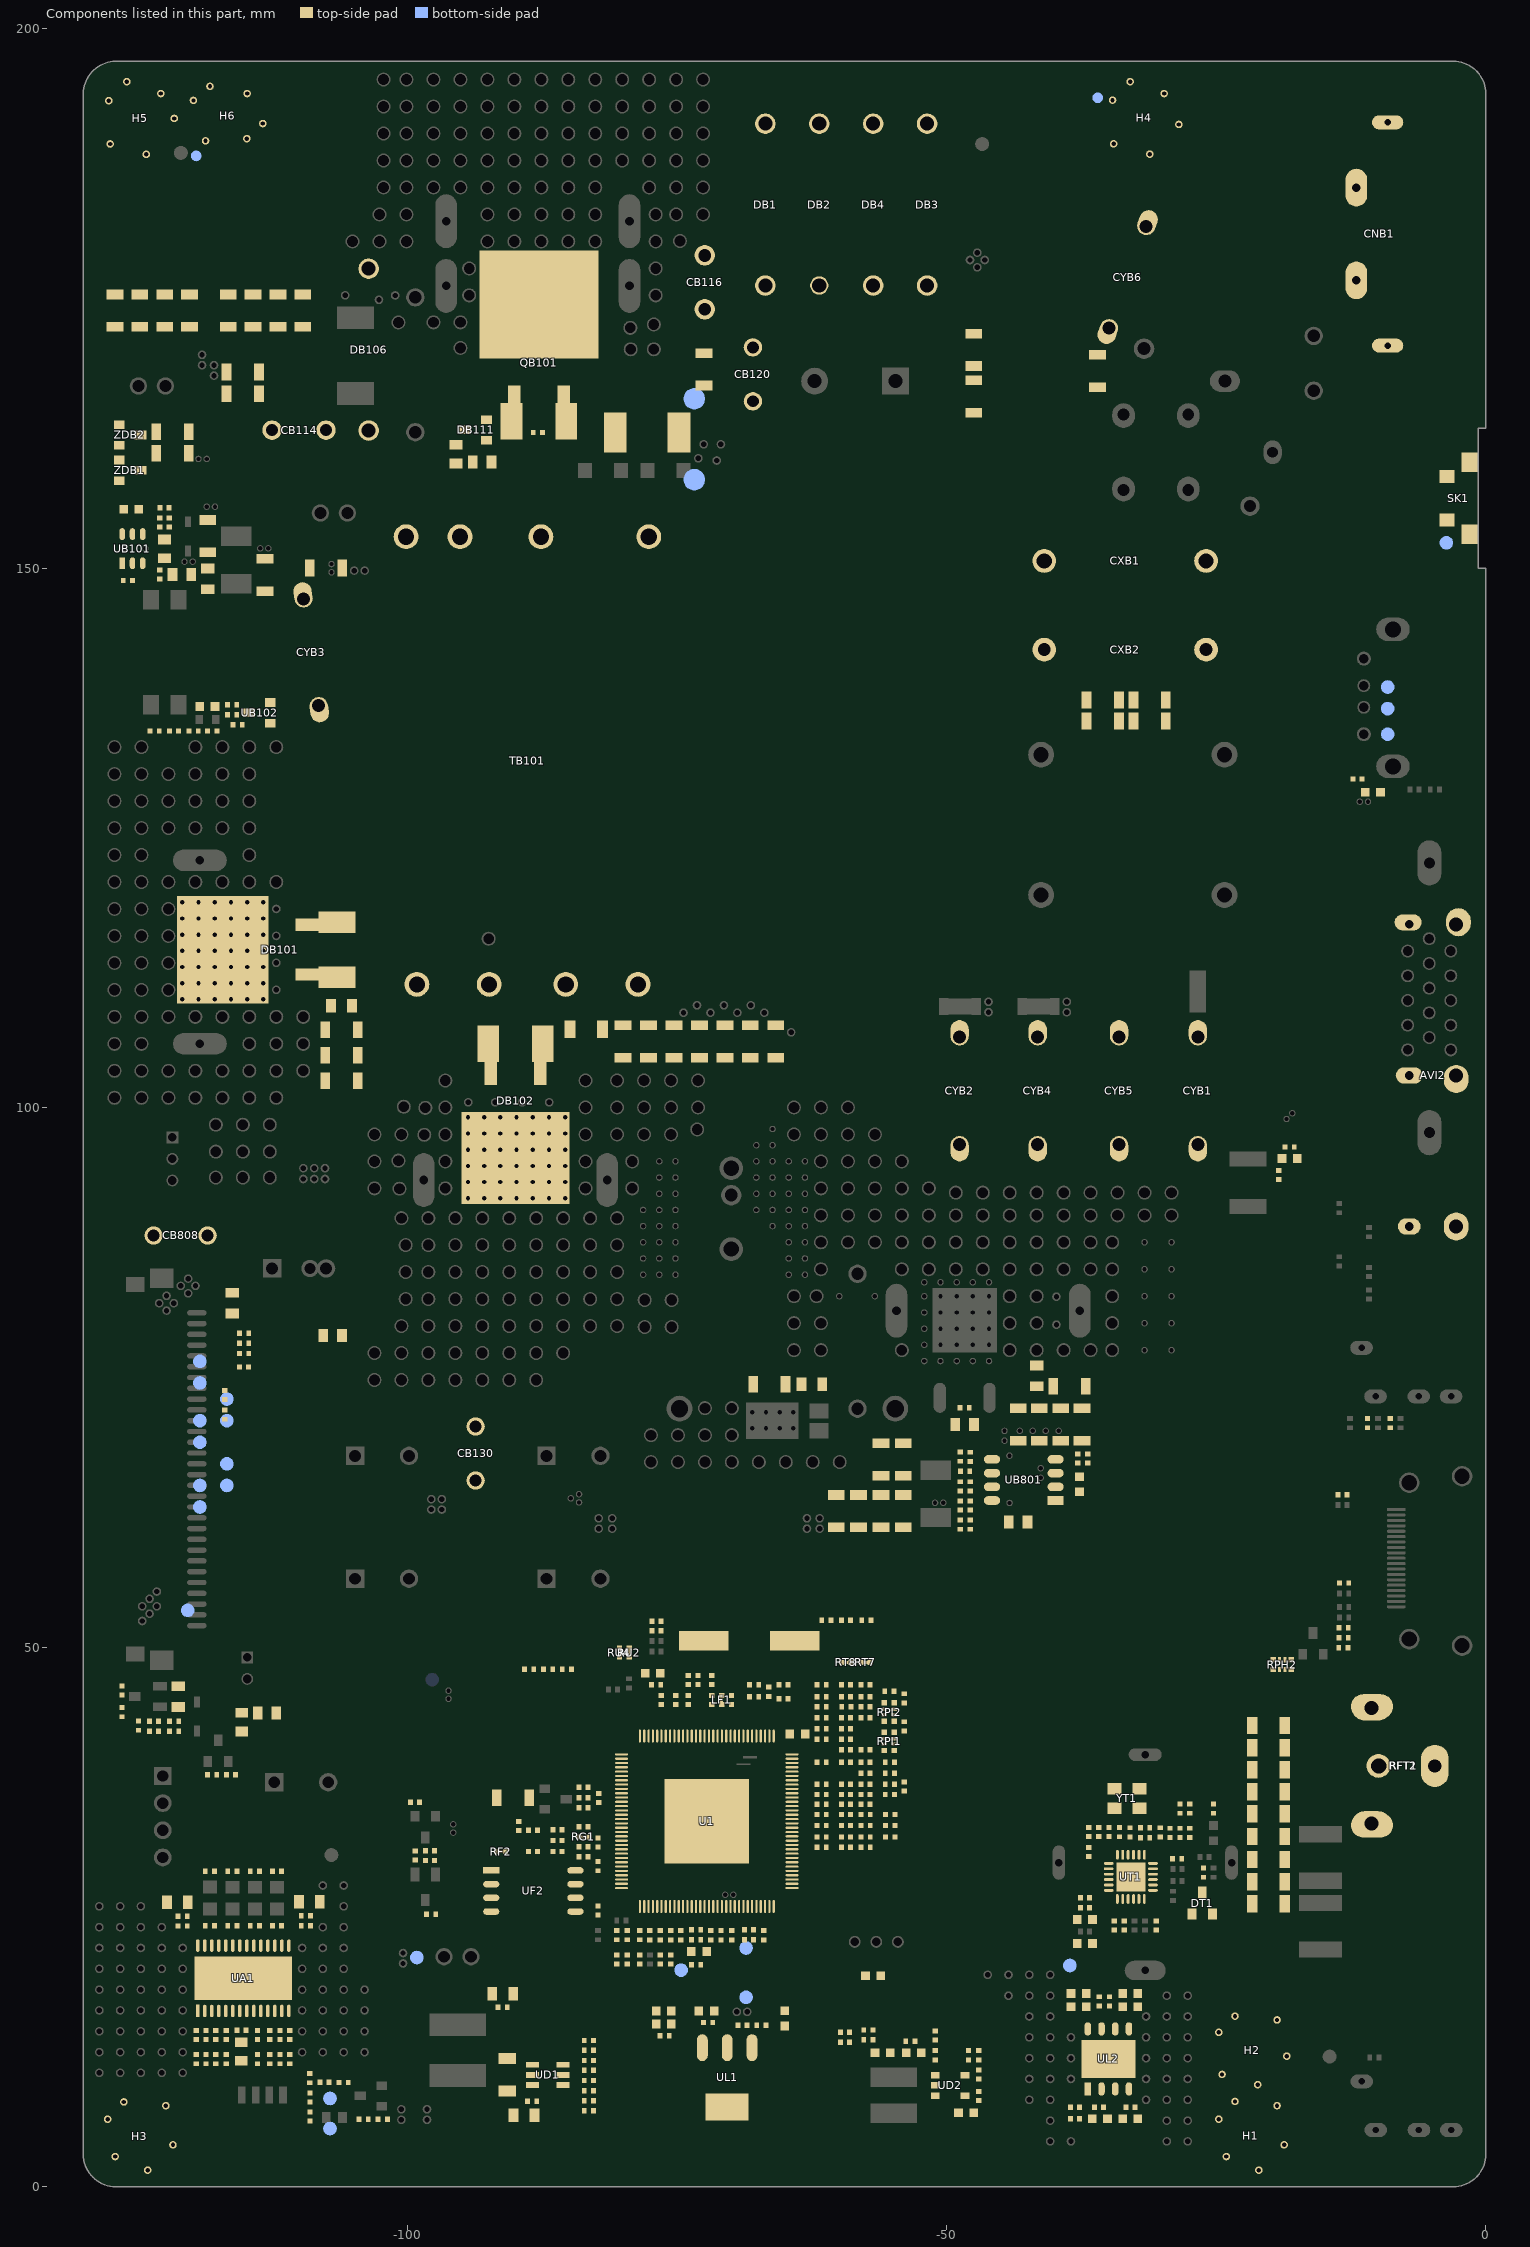
[diagram p0: the components of this part, seen from the top]
# Altium PCB MISC84438.PcbDoc (part 3 of 15)
Units mm, origin at the board's own origin, x right, y up, seen from the top; angles counter-clockwise.
Board outline 130 x 197 mm, 2 copper layers (TopLayer, BottomLayer), stack 1.571 mm thick; 574 components, 314 nets, 2636 pads, 811 vias.

## Components (designator, comment, footprint, x,y, rotation, side; value= is the part's Value field where it differs from the comment) (continued)
RB148 "Thick-film resistor,RES,2W,0.22ohm,±5%,2512,SMD" R2512-1 -77.737,162.59 r180 top
RB150 "150Kohm-1206-±5%-1/4W" R1206 -124.769,173.897 r270 top
RB151 "150Kohm-1206-±5%-1/4W" R1206 -122.469,173.897 r270 top
RB152 "150Kohm-1206-±5%-1/4W" R1206 -127.07,173.897 r270 top
RB153 "150Kohm-1206-±5%-1/4W" R1206 -114.266,173.897 r90 top
RB154 "150Kohm-1206-±5%-1/4W" R1206 -109.665,173.897 r90 top
RB155 "150Kohm-1206-±5%-1/4W" R1206 -111.966,173.897 r90 top
RB156 "NC/150Kohm-1206-±5%-1/4W" R1206 -120.168,173.897 r270 top
RB157 "NC/150Kohm-1206-±5%-1/4W" R1206 -116.567,173.897 r90 top
RB158 "NC/Thick-film resistor,RES,1/16W,51ohm,±1%,0402,SMD" R0402 -119.781,134.925 r0 top
RB162 "NC/68ohm-1206-±5%-1/4W" R1206 -68.173,106.143 r270 top
RB163 "NC/68ohm-1206-±5%-1/4W" R1206 -72.893,106.142 r270 top
RB164 "NC/68ohm-1206-±5%-1/4W" R1206 -77.613,106.142 r270 top
RB165 "NC/68ohm-1206-±5%-1/4W" R1206 -106.07,104.881 r180 top
RB803 "Thick-film resistor,RES,1/16W,18Kohm,±1%,0402,SMD" R0402 -48.73,63.132 r90 top
RB804 "NC/10Kohm-0402-±5%-1/16W" R0402 -48.26,66.294 r0 top
RB805 "100ohm-0402-±5%-1/16W" R0402 -48.73,67.666 r90 top
RB806 "Thick-film resistor,RES,1/16W,1Kohm,±1%,0402,SMD" R0402 -36.893,67.496 r90 top
RB807 "20ohm-0805-±5%-1/8W" R0805 -48.311,70.65 r180 top
RB808 "10Kohm-0402-±1%-1/16W" R0402 -48.311,72.2 r180 top
RB810 "Thick-film resistor,RES,1/4W,10ohm,±5%,1206,SMD" R1206 -38.593,74.18 r0 top
RB812 "Thick-film resistor,RES,1/4W,10ohm,±5%,1206,SMD" R1206 -66.416,74.364 r180 top
RB813 "100ohm-0402-±5%-1/16W" R0402 -48.73,61.366 r270 top
RB814 "Thick-film resistor,RES,1/4W,270Kohm,±1%,1206-Auto,SMD" R1206 -56.069,67.399 r270 top
RB816 "10ohm-0805-±5%-1/8W" R0805 -43.355,61.595 r0 top
RB818 "Thick-film resistor,RES,1/4W,0.2ohm,±1%,1206,SMD" R1206 -37.423,70.65 r270 top
RB819 "Thick-film resistor,RES,1/4W,0.2ohm,±1%,1206,SMD" R1206 -39.404,70.65 r270 top
RB820 "Thick-film resistor,RES,1/4W,0.2ohm,±1%,1206,SMD" R1206 -41.386,70.65 r270 top
RB821 "Thick-film resistor,RES,1/4W,0.2ohm,±1%,1206,SMD" R1206 -43.354,70.65 r270 top
RB835 "Thick-film resistor,RES,1/4W,270Kohm,±1%,1206-Auto,SMD" R1206 -53.993,67.399 r90 top
RB837 "Thick-film resistor,RES,1/4W,1.5ohm,±1%,1206,SMD" R1206 -60.221,62.611 r90 top
RB838 "Thick-film resistor,RES,1/4W,1.6ohm,±1%,1206,SMD" R1206 -58.145,62.611 r90 top
RB839 "Thick-film resistor,RES,1/4W,3.3ohm,±1%,1206,SMD" R1206 -56.069,62.611 r270 top
RB840 "NC/1R5ohm-1206-±1%-1/4W" R1206 -53.993,62.611 r90 top
RD2 "0ohm-0402-±5%-1/16W" R0402 -83.146,12.625 r0 top
RD6 "12K4ohm-0402-±1%-1/16W" R0402 -47.015,12.179 r90 top
RD7 "13Kohm-0402-±1%-1/16W" R0402 -47.015,10.389 r90 top
RD8 "68Kohm-0402-±1%-1/16W" R0402 -51.027,14.008 r270 top
RD13 "Thick-film resistor,RES,1/16W,330Kohm,±1%,0402,SMD" R0402 -83.146,10.771 r0 top
RD14 "100Kohm-0402-±5%-1/16W" R0402 -83.146,7.048 r180 top
RD15 "0ohm-0402-±5%-1/16W" R0402 -83.146,8.903 r0 top
RD16 "60K4ohm-0402-±1%-1/16W" R0402 -83.146,9.842 r180 top
RD88 "NC/1Mohm-0402-±5%-1/16W" R0402 -83.146,7.977 r180 top
RF1 "NC/1Mohm-0402-±5%-1/16W" R0402 -73.025,46.964 r270 top
RF2 "NC/0ohm-0402-PCB" R0402SC -91.3,31.064 r0 top
RF3 "4K7ohm-0402-±5%-1/16W" R0402 -82.296,25.603 r270 top
RF8 "4K7ohm-0402-±5%-1/16W" R0402 -80.543,21.054 r270 top
RF9 "4K7ohm-0402-±5%-1/16W" R0402 -79.578,21.054 r270 top
RF10 "100ohm-0402-±5%-1/16W" R0402 -79.578,23.314 r90 top
RF11 "100ohm-0402-±5%-1/16W" R0402 -80.543,23.314 r90 top
RF12 "180ohm-0402-±5%-1/16W" R0402 -55.245,39.345 r180 top
RF14 "NC/200Kohm-0402-±5%-1/16W" R0402 -57.233,13.602 r180 top
RF15 "NC/200Kohm-0402-±5%-1/16W" R0402 -59.405,14.313 r180 top
RF16 "NC/68ohm-0402-±5%-1/16W" R0402 -55.207,34.493 r0 top
RF19 "NC/68ohm-0402-±5%-1/16W" R0402 -59.309,37.313 r0 top
RF20 "NC/100ohm-0402-±5%-1/16W" R0402 -115.093,78.169 r0 top
RF21 "0ohm-0402-±5%-1/16W" R0402 -115.093,79.109 r180 top
RF22 "NC/4K7ohm-0402-±5%-1/16W" R0402 -115.118,75.972 r180 top
RF23 "NC/0ohm-0402-±5%-1/16W" R0402 -88.671,47.955 r180 top
RF24 "1Kohm-0402-±5%-1/16W" R0402 -61.125,52.489 r180 top
RF25 "NC/0ohm-0402-±5%-1/16W" R0402 -86.919,47.955 r180 top
RF26 "NC/4K7ohm-0402-±5%-1/16W" R0402 -115.093,77.229 r180 top
RF27 "NC/0ohm-0402-±5%-1/16W" R0402 -85.192,47.955 r180 top
RFT1 "NC/RF connector,RF JACK,H,F,T14.5,CH6.3,without pipe,12.4×13.2×7.7mm,DIP,LHD" T-13.2×12.4×7.7-F14.5 -4.45,39 r90 top locked
RFT2 "RF connector,RF JACK,H,IEC,T14.5,CH6.3,12.4×13.2×7.7mm,DIP,LHD-020 assembly,LHD" ANT-IEC14.5-H-4 -4.5,39 r90 top locked
RG1 "NC/0ohm-0402-PCB" R0402SC -83.642,32.41 r180 top
RH1 "0ohm-0402-±5%-1/16W" R0402 -13.284,64.135 r180 top
RH2 "0ohm-0402-±5%-1/16W" R0402 -66.916,23.302 r270 top
RH10 "22ohm-0402-±5%-1/16W" R0402 -70.891,23.302 r270 top
RH11 "22ohm-0402-±5%-1/16W" R0402 -71.831,23.302 r270 top
RH13 "220ohm-0402-±5%-1/16W" R0402 -69.913,23.302 r90 top
RH14 "1Kohm-0402-±5%-1/16W" R0402 -13.183,50.876 r180 top
RH28 "NC/10Kohm-0402-±5%-1/16W" R0402 -75.553,21.054 r270 top
RH29 "NC/15Kohm-0402-±1%-1/16W" R0402 -76.517,23.302 r270 top
RI2 "NC/150ohm-0402-±1%-1/16W" R0402 -57.506,36.346 r180 top
RI3 "NC/75ohm-0402-±5%-1/16W" R0402 -55.245,36.347 r0 top
RI8 "150ohm-0402-±1%-1/16W" R0402 -55.245,37.313 r180 top
RI9 "75ohm-0402-±5%-1/16W" R0402 -55.245,38.303 r0 top
RI13 "NC/0ohm-0402-±5%-1/16W" R0402 -53.899,45.262 r270 top
RI14 "NC/0ohm-0402-±5%-1/16W" R0402 -53.899,37.084 r270 top
RI15 "NC/0ohm-0402-±5%-1/16W" R0402 -53.899,42.672 r90 top
RK1 "NC/1K5ohm-0402-±5%-1/16W" R0402 -107.645,9.677 r180 top
RK3 "1Kohm-0402-±5%-1/16W" R0402 -76.517,21.054 r270 top
RK4 "12Kohm-0402-±1%-1/16W" R0402 -73.203,20.559 r0 top
RK6 "1K2ohm-0402-±1%-1/16W" R0402 -78.435,21.054 r90 top
RK13 "22ohm-0402-±5%-1/16W" R0402 -108.991,8.268 r90 top
RK15 "4K7ohm-0402-±5%-1/16W" R0402 -108.991,6.502 r270 top
RK16 "1Kohm-0402-±5%-1/16W" R0402 -88.316,31.064 r180 top
RK18 "NC/33Kohm-0402-±5%-1/16W" R0402 -89.637,33.426 r270 top
RK20 "NC/10Kohm-0402-±5%-1/16W" R0402 -102.248,6.248 r180 top
RK21 "510ohm-0402-±5%-1/16W" R0402 -104.013,6.248 r180 top
RL1 "NC/0ohm-0402-±5%-1/16W" R0402 -68.91,14.961 r0 top
RL2 "0ohm-0402-±5%-1/16W" R0402 -67.158,14.961 r0 top
RL4 "150ohm-0402-±1%-1/16W" R0402 -38.087,7.367 r0 top
RL5 "91ohm-0402-±1%-1/16W" R0402 -38.087,6.299 r0 top
RM1 "4K7ohm-0402-±5%-1/16W" R0402 -99.238,30.69 r270 top
RM2 "200Kohm-0402-±1%-1/16W" R0402 -97.866,31.147 r0 top
RM3 "10Kohm-0402-±5%-1/16W" R0402 -88.316,33.045 r180 top
RM4 "4K7ohm-0402-±5%-1/16W" R0402 -99.263,35.636 r0 top
RM5 "4K7ohm-0402-±5%-1/16W" R0402 -121.577,42.202 r0 top
RM6 "NC/4K7ohm-0402-±5%-1/16W" R0402 -124.892,42.735 r270 top
RM7 "47Kohm-0402-±5%-1/16W" R0402 -123.457,42.202 r180 top
RM8 "4K7ohm-0402-±5%-1/16W" R0402 -118.059,38.176 r180 top
RM10 "4K7ohm-0402-±5%-1/16W" R0402 -116.307,38.176 r0 top
RO1 "510ohm-0402-±5%-1/16W" R0402 -57.506,43.459 r0 top
RO2 "NC/100ohm-1206-±5%-1/4W" R1206 -90.17,36.043 r0 top
RO3 "NC/47Kohm-0402-±5%-1/16W" R0402 -57.506,45.416 r180 top
RO4 "NC/200Kohm-0402-±5%-1/16W" R0402 -59.309,43.459 r0 top
RO5 "510ohm-0402-±5%-1/16W" R0402 -59.284,44.475 r0 top
RO6 "NC/10Kohm-0402-±5%-1/16W" R0402 -83.642,36.065 r0 top
RO7 "NC/47Kohm-0402-±5%-1/16W" R0402 -59.309,46.507 r0 top
RO8 "NC/200Kohm-0402-±5%-1/16W" R0402 -61.57,45.416 r0 top
RO9 "NC/100ohm-0402-±5%-1/16W" R0402 -83.642,35.125 r0 top
RO10 "NC/1Kohm-0402-±5%-1/16W" R0402 -83.642,37.007 r0 top
RO12 "75ohm-0402-±5%-1/16W" R0402 -59.309,39.344 r180 top
RO13 "0ohm-0402-±5%-1/16W" R0402 -55.296,45.936 r180 top
RO14 "0ohm-0402-±5%-1/16W" R0402 -57.506,40.5 r180 top
RO15 "0ohm-0402-±5%-1/16W" R0402 -57.506,46.507 r180 top
RPH2 "Resistor array,RES ARRAY,1/16W,4×10Kohm,±5%,0402,SMD" RA0402 -18.872,48.387 r90 top
RPI1 "Resistor array,RES ARRAY,1/16W,4×10Kohm,±5%,0402,SMD" RA0402 -55.296,41.275 r0 top
RPI2 "NC/Resistor array,RES ARRAY,1/16W,4×10Kohm,±5%,0402,SMD" RA0402 -55.296,43.993 r0 top
RR1 "NC/0ohm-0402-±5%-1/16W" R0402 -83.642,30.582 r0 top
RT2 "100ohm-0402-±5%-1/16W" R0402 -36.804,32.88 r90 top
RT3 "4K7ohm-0402-±5%-1/16W" R0402 -76.879,52.417 r0 top
RT4 "4K7ohm-0402-±5%-1/16W" R0402 -76.879,51.515 r0 top
RT5 "33ohm-0402-±5%-1/16W" R0402 -28.347,35.039 r270 top
RT6 "33ohm-0402-±5%-1/16W" R0402 -27.432,35.039 r270 top
RT7 "NC/" R0402SC -57.506,48.59 r180 top
RT8 "NC/" R0402SC -59.309,48.59 r180 top
RT9 "NC/430ohm-0402-±5%-1/16W" R0402 -66.453,45.872 r90 top
RT11 "1K8ohm-0402-±5%-1/16W" R0402 -30.188,32.842 r270 top
RT18 "10Kohm-0402-±5%-1/16W" R0402 -35.89,32.868 r90 top
RU2 "NC/0ohm-0402-PCB" R0402SC -79.39,49.504 r270 top
RU4 "NC/0ohm-0402-PCB" R0402SC -80.305,49.504 r270 top
RV1 "NC/33ohm-0402-±5%-1/16W" R0402 -59.309,34.493 r0 top
RV2 "NC/75ohm-0402-±5%-1/16W" R0402 -57.48,34.493 r180 top
RV3 "NC/33ohm-0402-±5%-1/16W" R0402 -59.309,33.477 r0 top
RV5 "NC/75ohm-0402-±5%-1/16W" R0402 -55.207,33.476 r180 top
RV9 "NC/33ohm-0402-±5%-1/16W" R0402 -57.48,32.41 r0 top
RV10 "NC/100ohm-0402-±5%-1/16W" R0402 -59.309,35.433 r180 top
RV11 "NC/75ohm-0402-±5%-1/16W" R0402 -55.207,32.41 r180 top
RV12 "NC/100ohm-0402-±5%-1/16W" R0402 -59.309,31.445 r180 top
RV13 "NC/10Kohm-0402-±5%-1/16W" R0402 -57.48,31.445 r0 top
RV14 "NC/10Kohm-0402-±5%-1/16W" R0402 -57.506,35.433 r0 top
S/N1 "Barcode" Barcode -29.8,74.6 r270 bottom
S/N2 "Barcode" Barcode -57.912,47.879 r0 bottom
SK1 "Tact switch,Tact Switch,260±50gf,7.8×3.5×3.5mm,SMD,KFC-011SB-H3.5-EP,CS" KEY-HS-5 -0.703,156.5 r90 top locked
TB101 "Transformer,EQ2914,310uH,0.30×2P,29Ts,H14.5MAX,SYEQ2914Z-T012021A (BLACK),DIP,YX" T/EQ2914*9-1 -88.835,136.843 r270 top locked
TB-GND1 "NC/TEST" TP-10 -119.545,188.239 r90 bottom
TB-GND2 "NC/TEST" TP-10 -35.979,193.624 r90 bottom
TP-TDT "NC/" TP-TDT -73.368,161.976 r270 bottom
U1 "TV main chip,IC Main Chip,TSU69KR-Z1-ST,CH,32bit,Single-Core,LQFP128,SMD,Mstar" QFP128/0.4-5 -72.212,33.871 r90 top locked
UA1 "Audio amplifier,IC Audio AMP,Class D,2×10W@13.0V@8ohm,HTSSOP-28,SMD,RDA3118E28B,RDA" SSOP28/0.65-5 -115.175,19.315 r90 top
UB101 "PWM controller,IC PWM Controller,100KHz,SOT23-6,SMD,LD5523B GL,Leadtrend" SOT-26 -125.45,151.827 r180 top locked
UB102 "AZ431AN-ATRE1(BCD)" SOT-23-RAK -113.691,136.612 r90 top
UB801 "PWM controller,IC PWM Controller,120KHz,SOP-8,SMD,OB3353ACPA,ON-Bright" SO-8A -42.824,65.507 r180 top
UD1 "DC-DC chip,IC DCDC,Syn,2A,18V,500KHz,SOT23-6,SMD,LC2332CB6TR,Leadchip" SOT-23-6 -86.956,10.351 r270 top
UD2 "DC-DC chip,IC DCDC,Syn,1.2A,7.0V,1.5MHz,SOT23-5,SMD,LC2127CB5TR,Leadchip" SOT-23-5 -49.655,9.385 r270 top
UF2 "SPI FLASH chip,IC SPI FLASH,32Mb,SOIC8,SMD,GD25Q32CSIG,GigaDevice" SOIC8 -88.29,27.407 r0 top
UL1 "LC1117CLTR18" SOT-223 -70.323,10.127 r180 top
UL2 "LDO chip,IC LDO,1A,3.3V+ADJ,12V,ESOP-8,SMD,LC1118CS8TRAD33,Leadchip" SOP8/1.27-3 -34.989,11.836 r90 top
USB0_M "TEST" TP -9.096,137 r90 bottom
USB0_P "TEST" TP -9.096,139 r90 bottom
USB_5V "TEST" TP -9.096,134.63 r90 bottom
UT1 "Silicon tuner,IC Si Tuner,QFN24,SMD,R842,Rafael" QFN24/0.5-3 -32.906,28.714 r180 top locked
VCC_PANEL "TEST" TP -120.326,53.418 r90 bottom
XXXXXX "PCB_TIME" PCB_TIME -71.756,61.053 r90 top
XXXXXXXXXXXXXXX "PCB_NAME" PCB_NAME -67.793,58.272 r90 top
YF1 "Passive standard-package crystal oscillator,SPXO,24MHz,±20PPM,20pF,HC-49SMD,SMD,SD2024M00020T2115047,JWT" XTAL-S-1 -68.275,50.594 r180 top
YT1 "NC/Passive standard-package crystal oscillator,SPXO,24MHz,±20ppm,16pF,3.2×2.5,SMD,SMD3225 24.000MHZ,JWT" XTAL-S-10 -33.265,35.979 r0 top
ZDB1 "NC/BZX84C24 (Blue Rocket)" SO-23 -125.654,159.093 r90 top
ZDB2 "NC/Switching diode,DIO SW D1,215mA,85V,SOT-23,SMD,KAV70,KEXIN" SO-23 -125.654,162.369 r90 top
用于U1上方 "Glue,0.1g,silicone,ZJ" "Heat-Shrinkable Tube" -19.101,-1.88 r90 top

## Footprints (in the part's own frame and the unit in brackets; to place one, negate y for a bottom-side part, rotate by r counter-clockwise, add the part's x,y. Pads: shape width x height; smd on the part's side, far side on the other; paste and mask are expansions set on the pad)
AI_GRIPPER_V [mm] "3D shape for vertical type AI equipment"
  round 1.5 on Mech5: 0(0,-2.5) 1(0,0) 2(0,2.5)
  body extent -29.13,-4.7 2.5,4.7, height 54.74
ANT-IEC14.5-H-4 [mm] "联宏达；13.2×12.4×7.7mm LHD-020 中心高度6.3mm 160323(18.03.09更新脚距）,向内扩宽丝印,0703_2018（18.08.29 更新短槽孔）"
  oval 2.5x3.8 on Top Overlay paste-4 mask-4: 0(-5.35,6.1) 0(5.35,6.1)
  round 2.4 on Top Overlay: 0(0,5.45)
  oval 4.1x2.7 on Top Overlay paste-4 mask-4: 0(0,0.25)
  round 2.2 hole 1.4: 1(0,5.45)
  oval 2.3x3.6 hole 1.3 slot 2.6 at 90 deg: 2(-5.35,6.1) 4(5.35,6.1)
  oval 3.9x2.5 hole 1.2 slot 2.6 at 0 deg: 3(0,0.25)
  KeepOutLayer pour cut-out: 0,3.95 -0.574,4.064 -1.061,4.389 -1.386,4.876 -1.5,5.45 -1.5,5.45 -1.386,6.024 -1.061,6.511 -0.574,6.836 0,6.95 0,6.95 0.574,6.836 1.061,6.511 1.386,6.024 1.5,5.45 1.5,5.45 1.386,4.876 1.061,4.389 0.574,4.064 0,3.95
  silkscreen extent -6.3,0 6.3,7.9, body extent -7.55,-35.2 7.55,7.7, height 13.76
ASSE4.0C-3#1 [mm] "定位孔(顶底层上锡)(17.12.09更新过孔位置）"
  round 4 on Keep-Out mask+0: 0(0,0)
  round 1.2 on Top Paste: 1(-2.856,0.268) 1(-2.015,2.041) 1(-0.232,2.859) 1(1.66,2.339) 1(2.775,0.725)
  round 1.2 on Top Solder: 1(-2.856,0.268) 1(-2.015,2.041) 1(-0.232,2.859) 1(1.66,2.339) 1(2.775,0.725)
  round 0.7 hole 0.4: 1(-2.05,-2.214) 2(-2.75,1.25) 3(-1.25,2.9) 4(2.65,2.5) 5(3.304,-1.128) 6(0.964,-3.474)
ASSE4.0C-3#2 [mm] "定位孔(顶底层上锡)(17.12.09更新过孔位置）"
  round 4 on Keep-Out mask+0: 0(0,0)
  round 1.2 on Top Paste: 1(-2.856,0.268) 1(-2.36,-1.63) 1(-2.015,2.041) 1(-0.76,-2.766) 1(-0.232,2.859) 1(1.196,-2.607) 1(1.66,2.339) 1(2.592,-1.228) 1(2.775,0.725)
  round 1.2 on Top Solder: 1(-2.856,0.268) 1(-2.36,-1.63) 1(-2.015,2.041) 1(-0.76,-2.766) 1(-0.232,2.859) 1(1.196,-2.607) 1(1.66,2.339) 1(2.592,-1.228) 1(2.775,0.725)
  round 0.7 hole 0.4: 1(-2.45,-2.6) 2(-2.75,1.3) 3(-1.25,2.8) 4(2.65,2.45) 5(3.55,-0.9) 6(0.85,-3.55)
ASSE4.0C-3#3 [mm] "定位孔(顶底层上锡)(17.12.09更新过孔位置）"
  round 4 on Keep-Out mask+0: 0(0,0)
  round 1.2 on Top Paste: 1(-2.856,0.268) 1(-2.015,2.041) 1(-0.232,2.859) 1(1.66,2.339) 1(2.775,0.725)
  round 1.2 on Top Solder: 1(-2.856,0.268) 1(-2.015,2.041) 1(-0.232,2.859) 1(1.66,2.339) 1(2.775,0.725)
  round 0.7 hole 0.4: 1(-2.05,-2.214) 2(-2.75,1.25) 3(-1.25,2.85) 4(2.65,2.5) 5(3.304,-1.128) 6(0.964,-3.474)
ASSE4.0C-3#4 [mm] "定位孔(顶底层上锡)(17.12.09更新过孔位置）"
  round 4 on Keep-Out mask+0: 0(0,0)
  round 1.2 on Top Paste: 1(-2.856,0.268) 1(-2.36,-1.63) 1(-0.76,-2.766) 1(1.196,-2.607) 1(2.592,-1.228) 1(2.775,0.725)
  round 1.2 on Top Solder: 1(-2.856,0.268) 1(-2.36,-1.63) 1(-0.76,-2.766) 1(1.196,-2.607) 1(2.592,-1.228) 1(2.775,0.725)
  round 0.7 hole 0.4: 1(-2.5,-2.65) 2(-2.6,1.4) 3(-0.97,3.115) 4(2.179,2.015) 5(3.55,-0.85) 6(0.85,-3.6)
ASSE4.0C-3#5 [mm] "定位孔(顶底层上锡)(17.12.09更新过孔位置）"
  round 4 on Keep-Out mask+0: 0(0,0)
  round 1.2 on Top Paste: 1(-2.856,0.268) 1(-2.36,-1.63) 1(-0.76,-2.766) 1(1.196,-2.607) 1(2.592,-1.228) 1(2.775,0.725)
  round 1.2 on Top Solder: 1(-2.856,0.268) 1(-2.36,-1.63) 1(-0.76,-2.766) 1(1.196,-2.607) 1(2.592,-1.228)
  round 0.7 hole 0.4: 1(-2.513,-2.658) 2(-2.645,1.35) 3(-0.97,3.115) 4(2.179,2.015) 5(3.425,-0.291) 6(0.83,-3.623)
ASSE4.0C-3#6 [mm] "定位孔(顶底层上锡)(17.12.09更新过孔位置）"
  round 4 on Keep-Out mask+0: 0(0,0)
  round 1.2 on Top Paste: 1(-2.856,0.268) 1(-2.36,-1.63) 1(-0.76,-2.766) 1(1.196,-2.607) 1(2.592,-1.228) 1(2.775,0.725)
  round 1.2 on Top Solder: 1(-2.856,0.268) 1(-2.36,-1.63) 1(-0.76,-2.766) 1(1.196,-2.607) 1(2.592,-1.228) 1(2.775,0.725)
  round 0.7 hole 0.4: 1(-1.674,-2.364) 2(-2.797,1.38) 3(-1.262,2.686) 4(2.179,2.015) 5(3.63,-0.763) 6(2.156,-2.16)
AV3-H14-15 [mm] "宇球；RC075-F03L3BY-A; 中心高度：5.5mm;15.11.24;170401兼容物料，更新高度;170802加大接地脚焊盘（18.03.09更新孔距）"
  oval 2.8x2.5 on Top Overlay: 0(-14,2.75) 0(0,2.75) 0(14,2.75)
  oval 1.7x2.7 on Top Overlay: 0(-14,7.1) 0(0,7.1) 0(14,7.1)
  oval 1.5x2.119 / inner oval 1.5x2.5 / far side oval 1.5x2.5 hole 0.8 slot 1.8 at 90 deg: 1(-14,7.1)
  oval 2.6x2.3 hole 1.3 slot 1.6 at 0 deg: 2(-14,2.75)
  oval 1.5x2.5 hole 0.8 slot 1.8 at 90 deg: 3(0,7.1)
  oval 2.6x2.3 hole 1.3 slot 1.6 at 0 deg copper offset -0.33,0: 4(0,2.75)
  oval 1.5x2.5 hole 0.8 slot 1.8 at 90 deg copper offset 0.191,0.102: 5(14,7.1)
  oval 2.6x2.3 hole 1.3 slot 1.6 at 0 deg copper offset 0.203,-0.203: 6(14,2.75)
  silkscreen extent -20.3,0 20.3,7.8, body extent -20.1,-9 20.1,7.9, height 10.7
Barcode [mm]
  round 0.3 on Mech2: 0(0,0)
  silkscreen extent -14.62,-3.98 15.38,4.02
C0402 [mm] "片式电容"
  rect 0.45x0.5 smd mask+0.076: 1(-0.425,0) 2(0.425,0)
  silkscreen extent -0.88,-0.4 0.88,0.4, body extent -0.5,-0.25 0.5,0.25, height 0.5
C0603 [mm] "片式电容"
  rect 0.8x0.8 smd mask+0.076: 1(-0.706,0) 2(0.706,0)
  silkscreen extent -1.39,-0.55 1.39,0.55, body extent -0.8,-0.4 0.8,0.4, height 0.8
C0805 [mm] "片式电容"
  rect 0.9x1.25 smd mask+0.076: 1(-0.966,0) 2(0.966,0)
  silkscreen extent -1.73,-0.78 1.73,0.78, body extent -1,-0.62 1,0.63, height 1.25
C1206 [mm] "片式电容"
  rect 1x1.6 smd mask+0.076: 1(-1.5,-0.001) 2(1.5,0.001)
  silkscreen extent -2.39,-0.95 2.39,0.95, body extent -1.6,-0.8 1.6,0.8, height 1.3
CAP6.5*5-V-5-1 [mm] "TDK，CC45SL3DD680JYSNA，外K型引脚，AI，0713_2018"
  round 2.1 on Top Overlay: 0(-2.5,0) 0(2.5,0)
  round 1.9 hole 1.2 mask+0.051: 1(-2.5,0) 2(2.5,0)
  BottomLayer lines w0.6: -2.19,0.39 -2.238,0.42 -4.056,1.556 ; 2.89,0.31 2.92,0.262 2.977,0.171 4.056,-1.556 ; -2.5,0 -4.056,1.556 ; 2.5,0 2.647,-0.147 4.056,-1.556 ; -2.89,-0.31 -2.92,-0.262 -4.056,1.556 ; 2.19,-0.39 2.238,-0.42 2.489,-0.577 4.056,-1.556
  silkscreen extent -5.5,-2.5 5.5,2.5
CAP8*2.5-V-5 [mm] "C242G472J20A201(编带/法拉)"
  round 1.8 hole 1.1: 1(-2.5,0) 2(2.5,0)
  round 2 on Top Overlay: 1(-2.5,0) 1(2.5,0)
  BottomLayer lines w0.6: -2.956,-0.35 -4.056,1.556 ; -2.5,0 -4.056,1.556 ; -2.15,0.456 -4.056,1.556 ; 2.15,-0.456 2.425,-0.614 2.432,-0.618 2.827,-0.846 2.866,-0.869 4.056,-1.556 ; 2.5,0 2.644,-0.143 2.688,-0.188 2.701,-0.201 2.729,-0.229 2.767,-0.267 3.225,-0.725 3.251,-0.751 4.056,-1.556 ; 2.956,0.35 2.985,0.299 3.129,0.049 3.142,0.026 3.289,-0.229 3.311,-0.267 3.523,-0.633 3.54,-0.663 4.056,-1.556
  silkscreen extent -4,-1.25 4,1.25
CAP10*4.5-V-5#1 [mm] "YU102472M090DAND5H，陶瓷电容，17.12.22"
  round 1.7 hole 1.1: 1(-2.5,0) 2(2.5,0)
  round 1.9 on Top Overlay: 41(2.5,0) 42(-2.5,0)
  BottomLayer lines w0.6: -2.19,0.39 -2.238,0.42 -3.788,1.388 -4.056,1.556 ; 2.89,0.31 2.92,0.262 ; -2.5,0 -3.788,1.288 -4.056,1.556 ; 2.5,0 2.526,-0.026 2.58,-0.08 2.832,-0.332 2.863,-0.363 3.206,-0.706 3.568,-1.068 3.647,-1.147 3.736,-1.236 3.842,-1.342 4.056,-1.556 ; -2.89,-0.31 -2.92,-0.262 -3.236,0.243 -3.788,1.128 -4.056,1.556 ; 2.19,-0.39 2.238,-0.42 2.364,-0.499 2.44,-0.546 2.466,-0.562 2.494,-0.58 2.526,-0.6 2.58,-0.634 2.605,-0.649 2.832,-0.791 3.01,-0.902 3.455,-1.18 3.587,-1.263 3.647,-1.3 3.736,-1.356 3.842,-1.422 4.056,-1.556 ; 2.92,0.262 2.931,0.244 2.974,0.176 3.209,-0.201 3.311,-0.363 3.402,-0.51 3.647,-0.902 3.68,-0.955 3.736,-1.044 3.802,-1.149 3.842,-1.213 4.01,-1.483 4.056,-1.556 ; 2.92,0.262 2.92,0.262
  silkscreen extent -5.55,-2.25 5.55,2.25
CAP10*4.5-V-5#2 [mm] "YU102472M090DAND5H，陶瓷电容，17.12.22"
  round 1.7 hole 1.1: 1(-2.5,0) 2(2.5,0)
  round 1.9 on Top Overlay: 41(2.5,0) 42(-2.5,0)
  BottomLayer lines w0.6: -2.19,0.39 -4.056,1.556 ; 2.89,0.31 2.92,0.262 ; -2.5,0 -4.056,1.556 ; 2.5,0 3.642,-1.142 4.056,-1.556 ; -2.89,-0.31 -4.056,1.556 ; 2.19,-0.39 2.238,-0.42 ; 2.92,0.262 3.642,-0.893 4.056,-1.556 ; 2.92,0.262 2.92,0.262 ; 2.92,0.262 2.92,0.262 ; 2.238,-0.42 3.642,-1.297 4.056,-1.556 ; 2.238,-0.42 2.238,-0.42 ; 2.238,-0.42 2.238,-0.42
  silkscreen extent -5.55,-2.25 5.55,2.25
CAP10*4.5-V-5#3 [mm] "YU102472M090DAND5H，陶瓷电容，17.12.22"
  round 1.7 hole 1.1: 1(-2.5,0) 2(2.5,0)
  round 1.9 on Top Overlay: 41(2.5,0) 42(-2.5,0)
  BottomLayer lines w0.6: 2.89,0.31 2.92,0.262 4.056,-1.556 ; 2.5,0 3.336,-0.836 4.056,-1.556 ; 2.238,-0.42 2.904,-0.836 4.056,-1.556 ; 2.238,-0.42 2.19,-0.39 ; -2.19,0.39 -2.238,0.42 -4.056,1.556 ; -2.5,0 -2.564,0.063 -4.056,1.556 ; -2.89,-0.31 -2.92,-0.262 -3.084,0 -3.123,0.063 -4.056,1.556
  silkscreen extent -5.55,-2.25 5.55,2.25
CAP13*5-V-10-1 [mm] "Walsin;YU1AH471M060DAMD0H;160718（18.03.15  更新孔径）"
  oval 2.35x1.7 hole 1.2 copper offset -0.375,0: 1(-5,0)
  oval 2.35x1.7 hole 1.2 copper offset 0.375,0: 2(5,0)
  oval 2.55x1.9 on Top Overlay: 61(-5,0) 61(5,0)
  silkscreen extent -5.71,-3 5.81,3
CAP18*5*11.5-V-15 [mm] "PX104K3ID19H200D9R(凯励)；170406加宽至6.4mm，方便兼容宽体物料直接上件"
  round 2.2 hole 1.2: 1(-7.5,0) 2(7.5,0)
  round 2.4 on Top Overlay: 3(-7.5,0) 4(7.5,0)
  silkscreen extent -9.25,-3.2 9.25,3.2
CAP18*8.5-V-15 [mm] "PX334K3ID49H200D9R(凯励)(18.01.12更新孔径）(18.07.18 更新丝印框，加了公差）"
  round 2.2 hole 1.4: 1(-7.5,0) 2(7.5,0)
  round 2.4 on Top Overlay: 77(7.5,0) 78(-7.5,0)
  silkscreen extent -9.25,-4.45 9.25,4.45
CAUTION [mm]
  silkscreen extent -10.17,-3.72 12.33,4.08
COLD [mm]
CON2-H8.6-1 [mm] "输入插座（ST-A03-005DT8+M02）东莞阳琦电子;15.01.21"
  round 3.3 on Keep-Out: 0(-6.5,-4.7) 0(6.5,-4.7)
  oval 1.5x3.1 on Top Overlay: 1(-10.35,-3.4) 1(10.35,-3.4)
  oval 3.5x2 hole 0.8 slot 2.2 at 0 deg: 1(-4.3,-0.5) 2(4.3,-0.5)
  oval 3.7x2.2 on Top Overlay: 1(-4.3,-0.5) 1(4.3,-0.5)
  oval 1.3x2.9 hole 0.6 slot 2.2 at 90 deg: 3(10.35,-3.4) 4(-10.35,-3.4)
  silkscreen extent -11,-14 11,2.78
"Conformal Coating" [mm] "三防漆虚线框"
  round 0.3 on Mech2: 0(0,0)
CQC [mm]
D2-H-15#1 [mm] "GOOD-ARK;HER201G~HER208G;14-04-18"
  round 2.1 on Top Overlay: 15(-7.5,0) 16(7.5,0)
  round 1.9 hole 1.3: A(-7.5,0) K(7.5,0)
  BottomLayer lines w0.6: -7.404,0.643 -7.312,0.615 ; 7.404,0.643 7.312,0.615 5.3,0 ; -7.5,0 -5.3,0 ; 7.5,0 5.3,0 ; -7.404,-0.643 -7.312,-0.615 -5.3,0 ; 7.404,-0.643 7.312,-0.615 7.092,-0.548 6.985,-0.515 5.3,0 ; -7.312,0.615 -7.312,0.615 ; -7.312,0.615 -5.3,0
  silkscreen extent -7.5,-1.8 7.5,1.8
D2-H-15#2 [mm] "GOOD-ARK;HER201G~HER208G;14-04-18"
  round 2.1 on Top Overlay: 15(-7.5,0) 16(7.5,0)
  round 1.9 hole 1.3: A(-7.5,0)
  round 1.7 / inner round 1.9 / far side round 1.9 hole 1.3: K(7.5,0)
  BottomLayer lines w0.6: 7.404,-0.643 7.312,-0.615 7.055,-0.536 6.625,-0.405 5.3,0 ; -7.404,-0.643 -7.345,-0.625 -7.312,-0.615 -5.749,-0.137 -5.685,-0.118 -5.3,0 ; 7.5,0 7.398,0 7.246,0 7.182,0 7.095,0 5.3,0 ; -7.5,0 -5.3,0 ; 7.404,0.643 7.398,0.642 7.312,0.615 ; -7.404,0.643 -7.312,0.615 ; 5.3,0 6.828,0.467 7.182,0.576 7.246,0.595 7.312,0.615 ; -5.3,0 -7.279,0.605 -7.312,0.615 ; 7.312,0.615 7.312,0.615 ; 7.312,0.615 7.312,0.615 ; -7.312,0.615 -7.312,0.615
  silkscreen extent -7.5,-1.8 7.5,1.8
D2-H-15#3 [mm] "GOOD-ARK;HER201G~HER208G;14-04-18"
  round 2.1 on Top Overlay: 15(-7.5,0) 16(7.5,0)
  round 1.9 hole 1.3: A(-7.5,0) K(7.5,0)
  BottomLayer lines w0.6: -7.404,0.643 -7.312,0.615 ; 7.404,0.643 7.351,0.627 7.312,0.615 6.985,0.515 6.732,0.438 5.612,0.095 5.449,0.046 5.3,0 ; -7.5,0 -5.3,0 ; 7.5,0 7.368,0 7.304,0 7.152,0 7.05,0 6.866,0 6.724,0 5.707,0 5.463,0 5.3,0 ; -7.404,-0.643 -7.312,-0.615 ; 7.404,-0.643 7.312,-0.615 7.188,-0.577 6.732,-0.438 6.64,-0.41 6.499,-0.367 6.391,-0.333 5.987,-0.21 5.48,-0.055 5.3,0 ; -7.312,0.615 -5.3,0 ; -7.312,0.615 -7.312,0.615 ; -5.3,0 -6.985,-0.515 -7.312,-0.615 ; -7.312,-0.615 -7.312,-0.615
  silkscreen extent -7.5,-1.8 7.5,1.8
D2-H-15#4 [mm] "GOOD-ARK;HER201G~HER208G;14-04-18"
  round 2.1 on Top Overlay: 15(-7.5,0) 16(7.5,0)
  round 1.9 hole 1.3: A(-7.5,0) K(7.5,0)
  BottomLayer lines w0.6: 7.404,-0.643 7.398,-0.642 7.312,-0.615 ; -7.404,-0.643 -7.312,-0.615 ; 7.5,0 6.073,0 5.971,0 5.819,0 5.755,0 5.3,0 ; -7.5,0 -5.3,0 ; 7.404,0.643 7.312,0.615 6.413,0.34 6.267,0.296 6.047,0.228 5.956,0.2 5.3,0 ; -7.404,0.643 -7.345,0.625 ; 7.312,-0.615 7.312,-0.615 ; 7.312,-0.615 7.312,-0.615 ; 7.312,-0.615 7.246,-0.595 7.182,-0.576 5.3,0 ; -7.312,-0.615 -7.312,-0.615 ; -7.312,-0.615 -7.307,-0.614 ; -7.307,-0.614 -7.307,-0.614 ; -7.307,-0.614 -7.279,-0.605 -6.138,-0.256 -6.083,-0.239 -6.038,-0.226 -5.3,0 ; -5.3,0 -5.358,0.018 -7.312,0.615 -7.317,0.617 ; -7.317,0.617 -7.317,0.617 ; -7.317,0.617 -7.345,0.625 ; -7.345,0.625 -7.345,0.625
  silkscreen extent -7.5,-1.8 7.5,1.8
D2-H-15#5 [mm] "GOOD-ARK;HER201G~HER208G;14-04-18"
  round 2.1 on Top Overlay: 15(-7.5,0) 16(7.5,0)
  round 1.9 hole 1.3: A(-7.5,0) K(7.5,0)
  BottomLayer lines w0.6: 7.404,-0.643 7.312,-0.615 7.15,-0.565 5.3,0 ; -7.404,-0.643 -7.312,-0.615 -7.252,-0.597 -6.787,-0.455 -6.443,-0.349 -5.943,-0.196 -5.764,-0.142 -5.745,-0.136 -5.591,-0.089 -5.3,0 ; 7.5,0 7.419,0 7.368,0 6.858,0 6.823,0 5.3,0 ; -7.5,0 -6.242,0 -5.817,0 -5.745,0 -5.3,0 ; 7.404,0.643 7.32,0.618 7.312,0.615 ; -7.404,0.643 -7.312,0.615 -6.175,0.268 -5.745,0.136 -5.649,0.107 -5.604,0.093 -5.306,0.002 ; 5.3,0 6.595,0.396 6.624,0.405 6.884,0.484 6.923,0.496 7.269,0.602 7.312,0.615 ; -5.3,0 -5.306,0.002 ; -5.306,0.002 -5.306,0.002 ; 7.312,0.615 7.312,0.615 ; 7.312,0.615 7.312,0.615 ; 7.312,0.615 7.312,0.615
  silkscreen extent -7.5,-1.8 7.5,1.8
D2PAK3#1 [mm] "伟达电子；SFS1006G;增加TO-252兼容；160309"
  rect 2x3.4 smd paste-5 mask-5: 1(-2.54,-10.6) 3(2.54,-10.6)
  rect 1.143x2.794 smd: 1(-2.3,-8.15) 3(2.3,-8.15)
  rect 6x6 smd: 2(0,-0.95)
  rect 10x8.5 smd paste-11 mask-11: 2(0,0)
  silkscreen extent -5.79,-7.95 5.79,4.54, body extent -5.25,-11.89 5.25,3.8, height 4.7